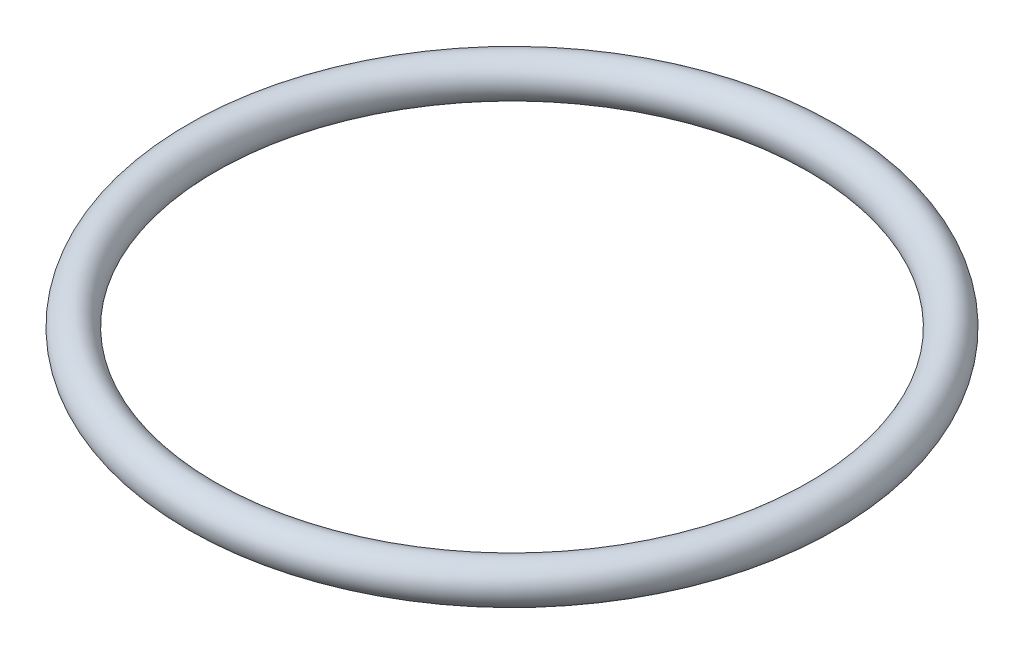
SolidWorks part; units mm, degrees
ref_plane "前视基准面" through (0, 0, 0) normal (0, 0, 1) x (1, 0, 0)
ref_plane "上视基准面" through (0, 0, 0) normal (0, 1, 0) x (1, 0, 0)
ref_plane "右视基准面" through (0, 0, 0) normal (1, 0, 0) x (0, 0, -1)
sketch "草图1" plane through (0, 0, 0) normal (0, 0, 1) x (1, 0, 0)
  line L0 (0, 0) -> (0, 14.5423) construction
  circle A0 centre (-36.125, 0) radius 2.25
  dimension "D1" = 36.125
  dimension "D2" = 4.5
revolve "旋转1" add sketch "草图1" angle 360 about L0
sketch "草图2" plane through (0, 0, 0) normal (0, 1, 0) x (1, 0, 0)
  circle A0 centre (0, 0) radius 36.8488
